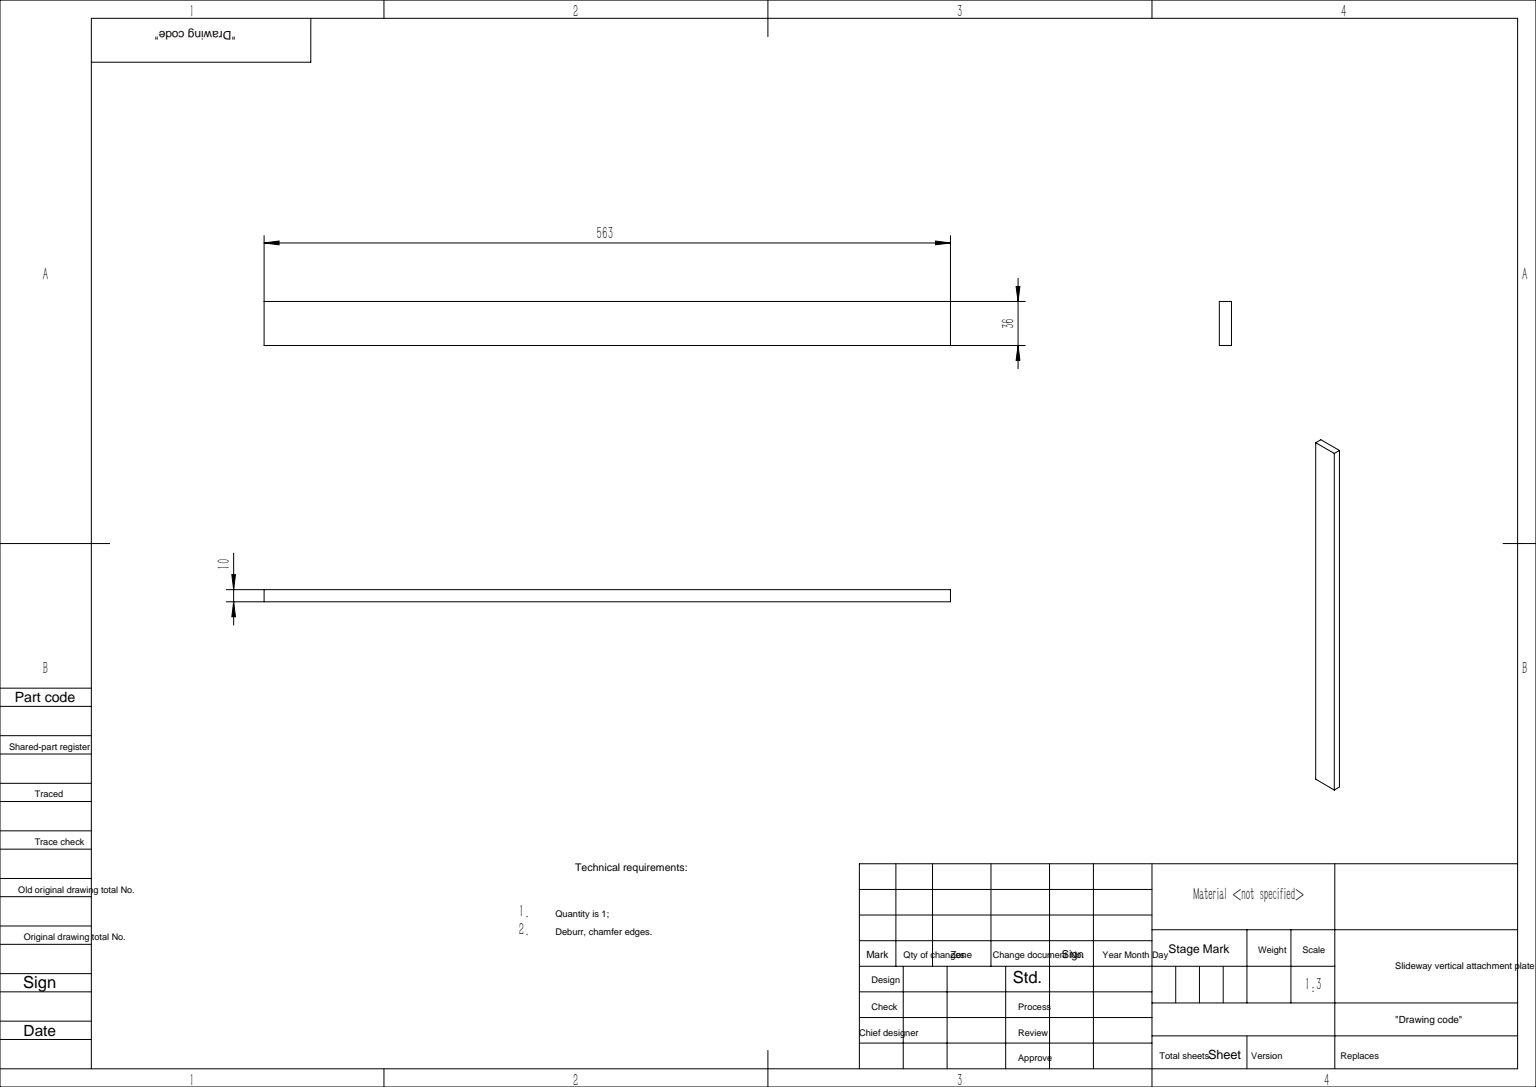
from build123d import *

# Parameters (mm, degrees)
SKETCH_1_W      = 36
SKETCH_1_H      = 10
EXTRUDE_1_DEPTH = 563


with BuildPart() as part:
    # 草图1 → 凸台-拉伸1 (new body)
    with BuildSketch(Plane(origin=(0, 30, 0), x_dir=(1, 0, 0), z_dir=(0, 1, 0))):
        with Locations((0, 15)):
            Rectangle(SKETCH_1_W, SKETCH_1_H)
    extrude(amount=EXTRUDE_1_DEPTH)


solid = part.part
